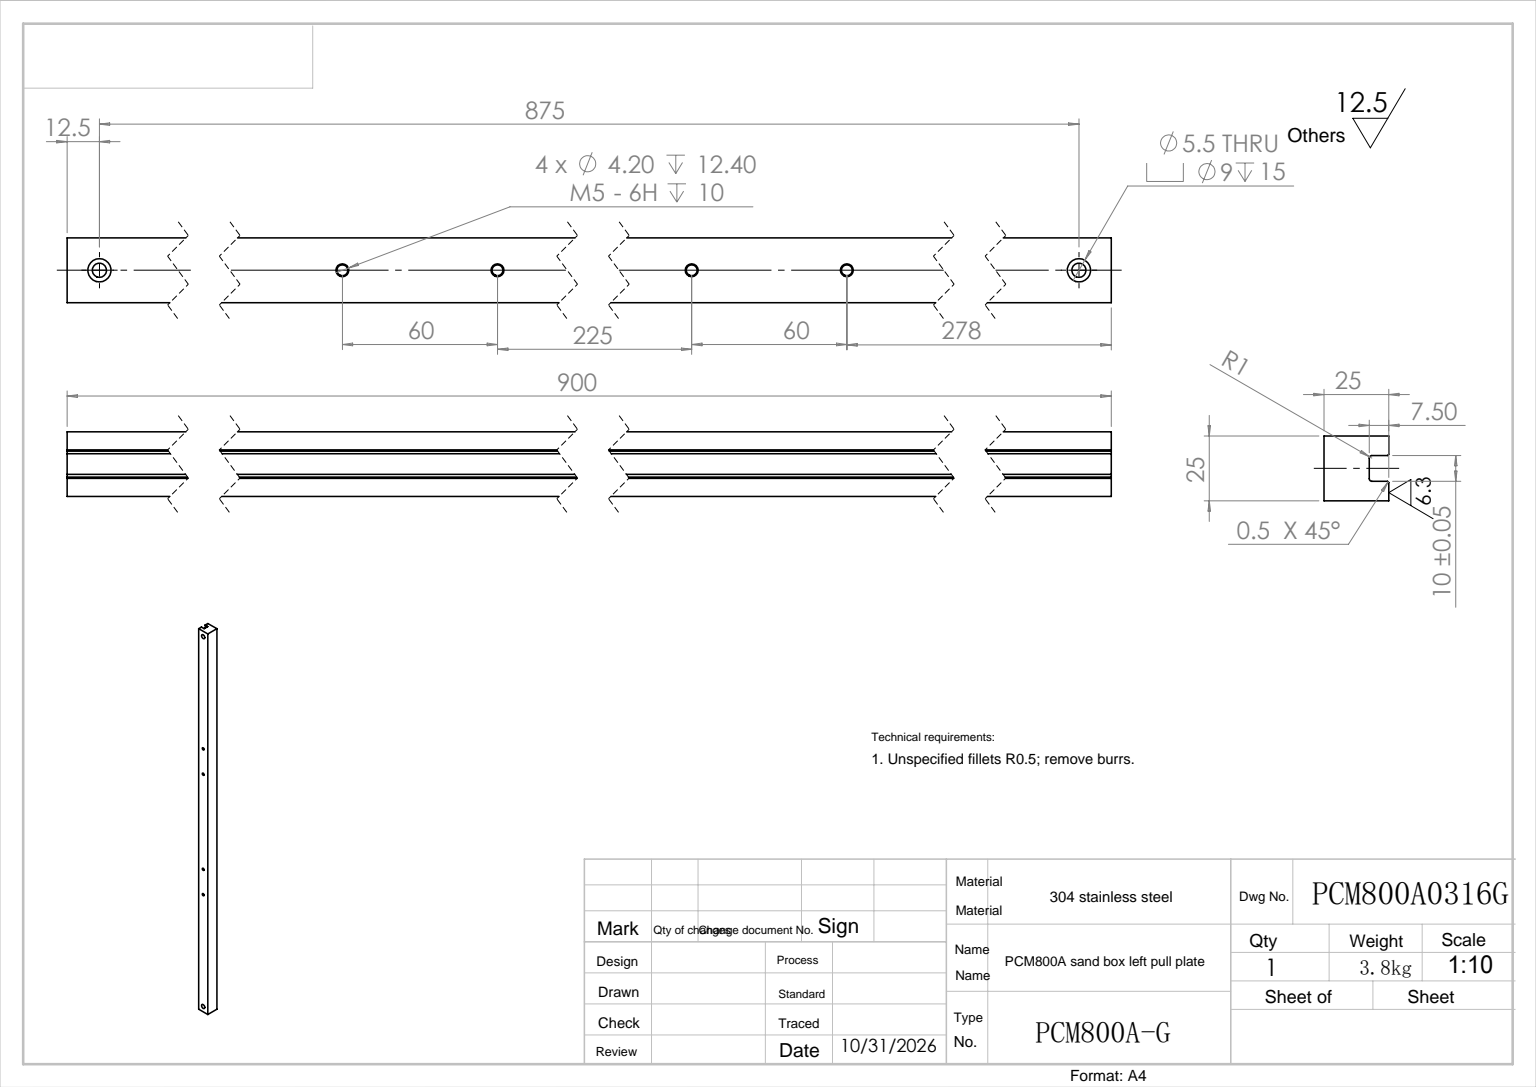
from build123d import *

# Parameters (mm, degrees)
SKETCH_1_W                  = 25
SKETCH_1_H                  = 900
EXTRUDE_1_DEPTH             = 25
CUT_EXTRUDE_1_DEPTH         = 901.694176733
CHAMFER_1_SIZE              = 0.5
HOLE_WIZARD_1_D             = 5.5
HOLE_WIZARD_1_CBORE_D       = 9
HOLE_WIZARD_1_CBORE_DEPTH   = 15
HOLE_WIZARD_M5_1_AT_2_COUNT = 2
HOLE_WIZARD_M5_1_AT_2_PITCH = 60
PATTERN_LINEAR_1_COUNT      = 2
PATTERN_LINEAR_1_PITCH      = 285


with BuildPart() as part:
    # 草图1 → 拉伸1 (new body)
    with BuildSketch(Plane(origin=(0, 0, 0), x_dir=(0, 0, -1), z_dir=(1, 0, 0))):
        with Locations((12.5, 450)):
            Rectangle(SKETCH_1_W, SKETCH_1_H)
    extrude(amount=EXTRUDE_1_DEPTH)

    # 草图2 → 切除-拉伸1 (cut, through all)
    with BuildSketch(Plane.XZ):
        with BuildLine():
            Line((0, -7.5), (6.5, -7.5))
            ThreePointArc((6.5, -7.5), (7.207106781, -7.792893219), (7.5, -8.5))
            Line((7.5, -8.5), (7.5, -16.5))
            ThreePointArc((7.5, -16.5), (7.207106781, -17.207106781), (6.5, -17.5))
            Line((6.5, -17.5), (0, -17.5))
            Line((0, -17.5), (0, -7.5))
        make_face()
    extrude(amount=-CUT_EXTRUDE_1_DEPTH, mode=Mode.SUBTRACT)

    # 倒角1
    chamfer_1_edges = [part.edges().sort_by_distance(p)[0] for p in [
        (0, 450, -17.5),
        (0, 450, -7.5),
    ]]
    chamfer(chamfer_1_edges, length=CHAMFER_1_SIZE)

    # 孔1 (through all)
    with Locations(Plane(origin=(12.5, 887.5, 0), x_dir=(1, 0, 0), z_dir=(0, 0, 1))):
        with Locations((0, 0), (0, -875)):
            CounterBoreHole(HOLE_WIZARD_1_D / 2, HOLE_WIZARD_1_CBORE_D / 2, HOLE_WIZARD_1_CBORE_DEPTH)

    # 草图5 → M5 螺纹孔1 (revolve, cut)
    with BuildSketch(Plane(origin=(12.5, 622, 0), x_dir=(0, -1, 0), z_dir=(1, 0, 0))):
        Polygon((0, 0), (0, 13.6618073), (2.1, 12.4), (2.1, 10), (2.5, 10), (2.5, 0), align=None)
    hole_wizard_m5_1 = revolve(axis=Axis((12.5, 622, 6.35), (0, 0, -1)), mode=Mode.SUBTRACT)

    # M5 螺纹孔1 at 2: M5 螺纹孔1 ×2
    with Locations(*[(0, -i * HOLE_WIZARD_M5_1_AT_2_PITCH, 0) for i in range(1, HOLE_WIZARD_M5_1_AT_2_COUNT)]):
        add(hole_wizard_m5_1, mode=Mode.SUBTRACT)

    # 阵列(线性)1: M5 螺纹孔1 ×2
    with Locations(*[(0, -i * PATTERN_LINEAR_1_PITCH, 0) for i in range(1, PATTERN_LINEAR_1_COUNT)]):
        add(hole_wizard_m5_1, mode=Mode.SUBTRACT)

    # 阵列(线性)1 copy 1 sketch → 阵列(线性)1 copy 1 (revolve, cut)
    with BuildSketch(Plane(origin=(12.5, 277, 0), x_dir=(0, -1, 0), z_dir=(1, 0, 0))):
        Polygon((0, 0), (0, 13.6618073), (2.1, 12.4), (2.1, 10), (2.5, 10), (2.5, 0), align=None)
    revolve(axis=Axis((12.5, 277, 6.35), (0, 0, -1)), mode=Mode.SUBTRACT)


solid = part.part
